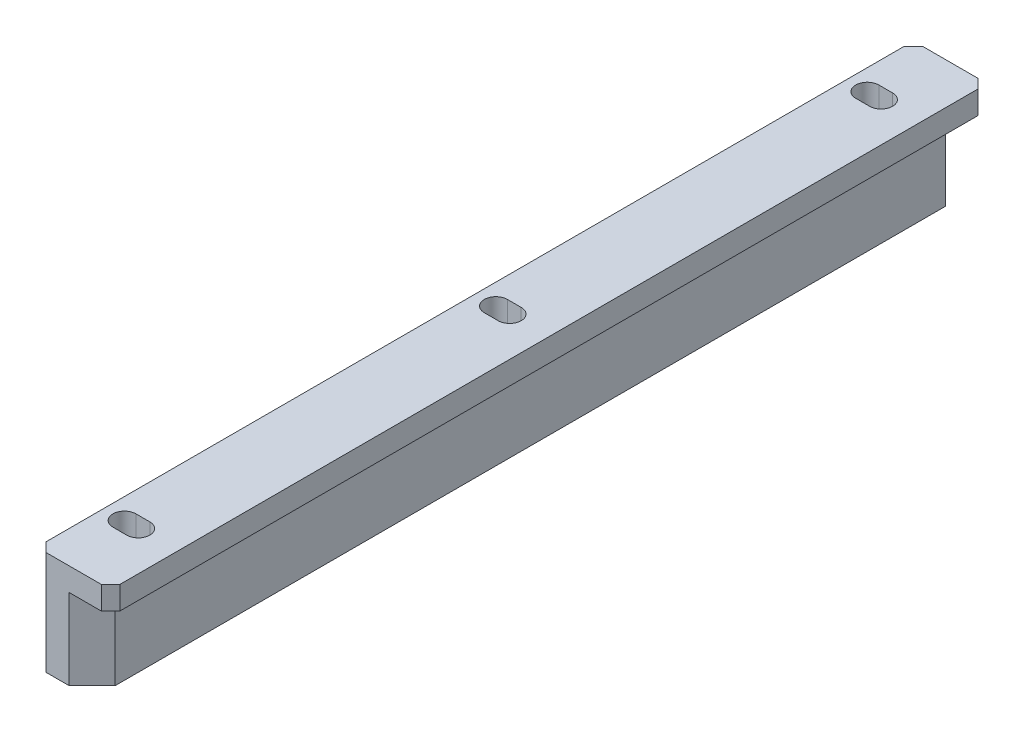
from build123d import *

# Parameters (mm, degrees)
EXTRUDE_1_DEPTH     = 95
CHAMFER_1_SIZE      = 5
CHAMFER_2_SIZE      = 2
CUT_EXTRUDE_1_REACH = 100.931


with BuildPart() as part:
    # 草图1 → 凸台-拉伸1 (new, symmetric)
    with BuildSketch(Plane.XY):
        Polygon((0, 0), (0, 22.5), (16, 22.5), (16, 17.5), (12, 17.5), (12, 0), align=None)
    extrude(amount=EXTRUDE_1_DEPTH, both=True)

    # 倒角1
    chamfer_1_edges = [part.edges().sort_by_distance(p)[0] for p in [
        (12, 8.75, 95),
        (12, 8.75, -95),
    ]]
    chamfer(chamfer_1_edges, length=CHAMFER_1_SIZE)

    # 倒角2
    chamfer_2_edges = [part.edges().sort_by_distance(p)[0] for p in [
        (16, 20, 95),
        (0, 11.25, 95),
        (0, 11.25, -95),
        (16, 20, -95),
    ]]
    chamfer(chamfer_2_edges, length=CHAMFER_2_SIZE)

    # 草图2 → 切除-拉伸1 (cut, up to next)
    with BuildSketch(Plane.XZ, mode=Mode.PRIVATE) as cut_extrude_1_sk1:
        with BuildLine():
            Line((4.5, 83), (7.5, 83))
            ThreePointArc((7.5, 83), (10, 80.5), (7.5, 78))
            Line((7.5, 78), (4.5, 78))
            ThreePointArc((4.5, 78), (2, 80.5), (4.5, 83))
        make_face()
    cut_extrude_1_tool1 = extrude(cut_extrude_1_sk1.sketch, amount=-CUT_EXTRUDE_1_REACH, mode=Mode.PRIVATE) & part.part
    # 草图2 → 切除-拉伸1 (cut, up to next)
    with BuildSketch(Plane.XZ, mode=Mode.PRIVATE) as cut_extrude_1_sk2:
        with BuildLine():
            Line((4.5, 2.5), (7.5, 2.5))
            ThreePointArc((7.5, 2.5), (10, 0), (7.5, -2.5))
            Line((7.5, -2.5), (4.5, -2.5))
            ThreePointArc((4.5, -2.5), (2, 0), (4.5, 2.5))
        make_face()
    cut_extrude_1_tool2 = extrude(cut_extrude_1_sk2.sketch, amount=-CUT_EXTRUDE_1_REACH, mode=Mode.PRIVATE) & part.part
    # 草图2 → 切除-拉伸1 (cut, up to next)
    with BuildSketch(Plane.XZ, mode=Mode.PRIVATE) as cut_extrude_1_sk3:
        with BuildLine():
            Line((4.5, -83), (7.5, -83))
            ThreePointArc((7.5, -83), (10, -80.5), (7.5, -78))
            Line((7.5, -78), (4.5, -78))
            ThreePointArc((4.5, -78), (2, -80.5), (4.5, -83))
        make_face()
    cut_extrude_1_tool3 = extrude(cut_extrude_1_sk3.sketch, amount=-CUT_EXTRUDE_1_REACH, mode=Mode.PRIVATE) & part.part
    add(cut_extrude_1_tool1.solids().sort_by_distance((6, 0, 80.5))[0], mode=Mode.SUBTRACT)
    add(cut_extrude_1_tool2.solids().sort_by_distance((6, 0, 0))[0], mode=Mode.SUBTRACT)
    add(cut_extrude_1_tool3.solids().sort_by_distance((6, 0, -80.5))[0], mode=Mode.SUBTRACT)


solid = part.part
